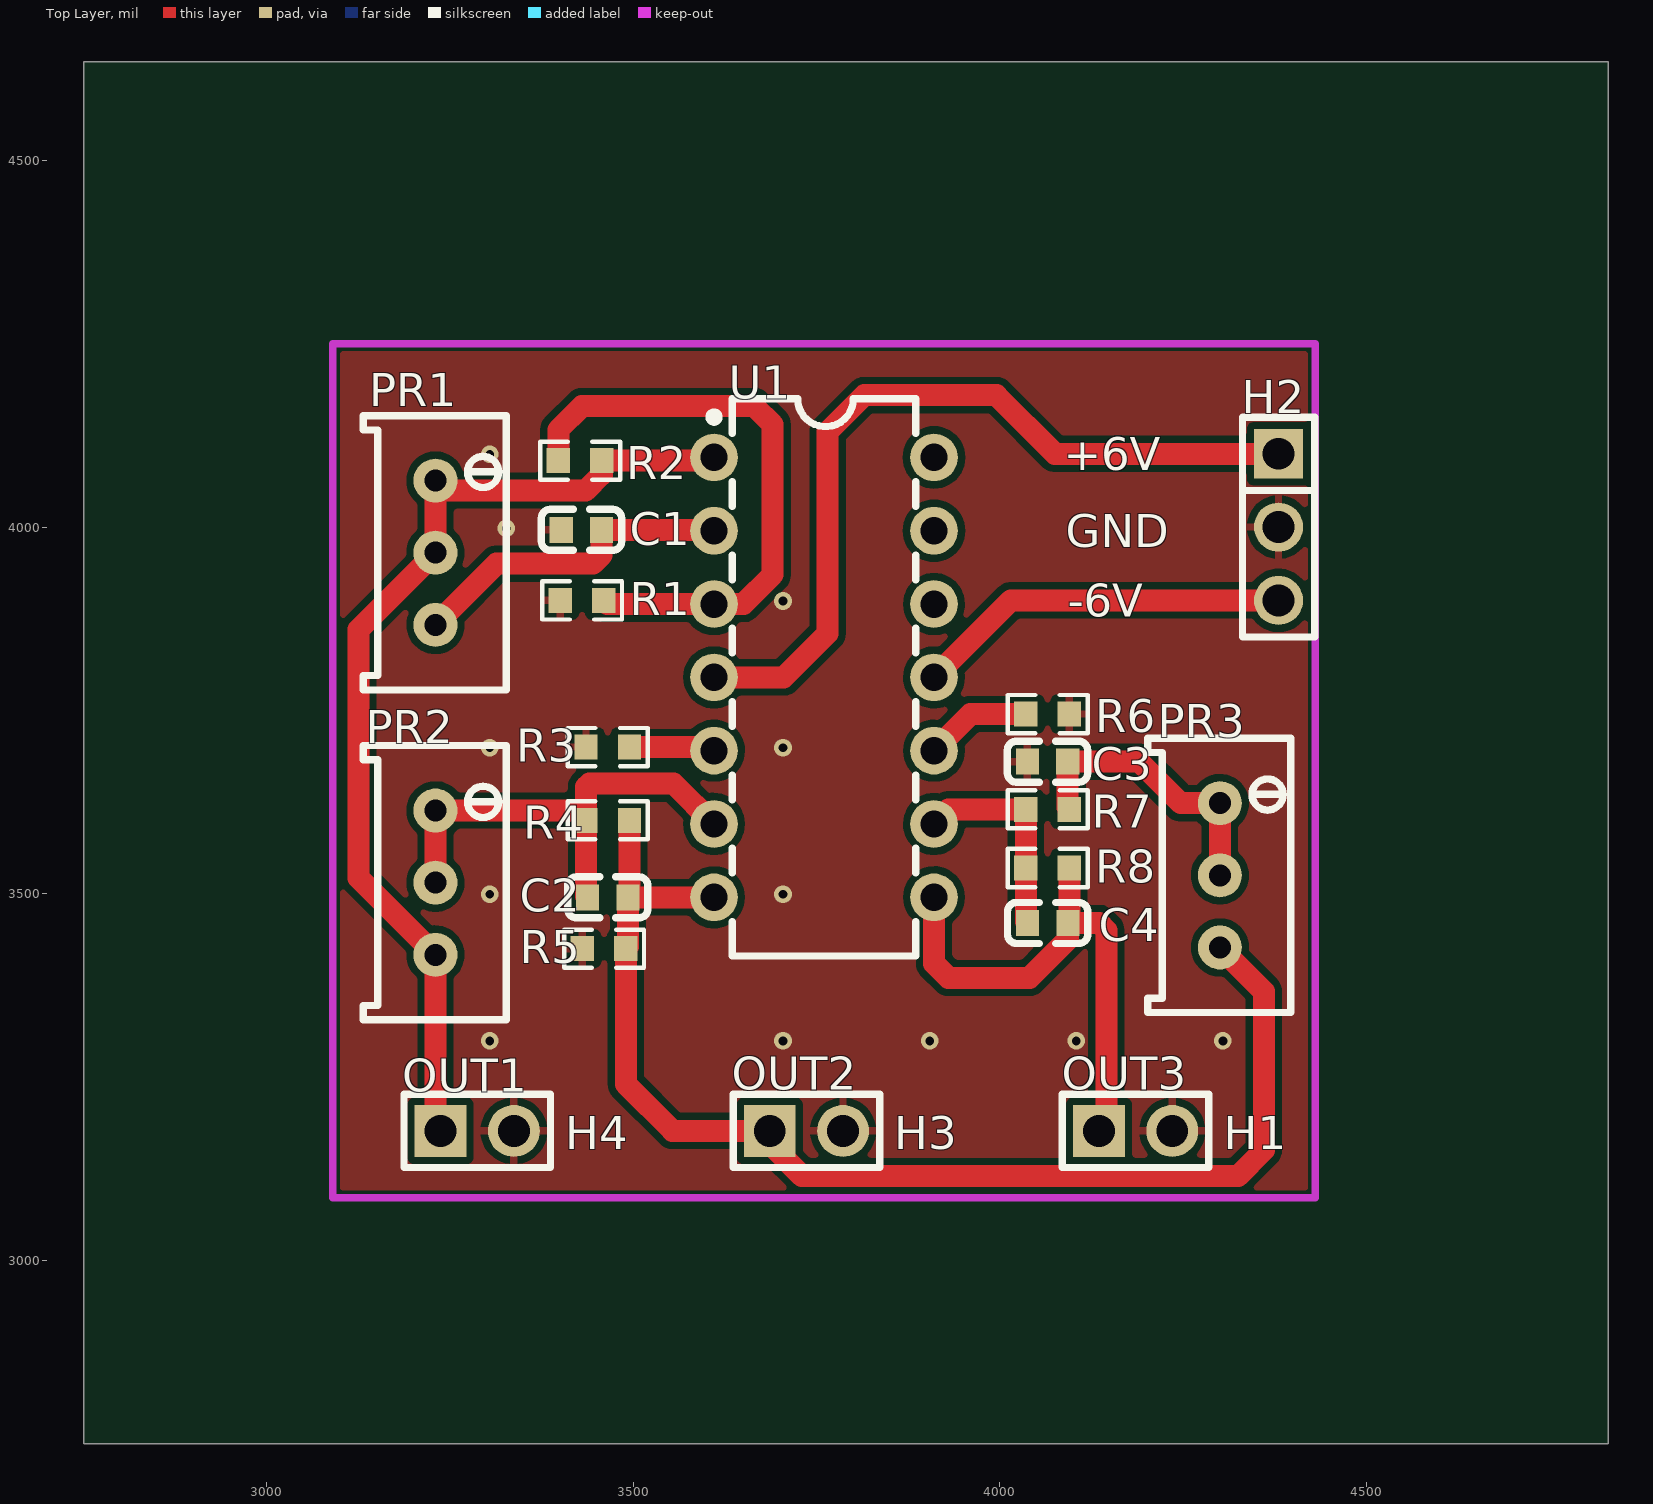
[diagram p0: Top Layer view]
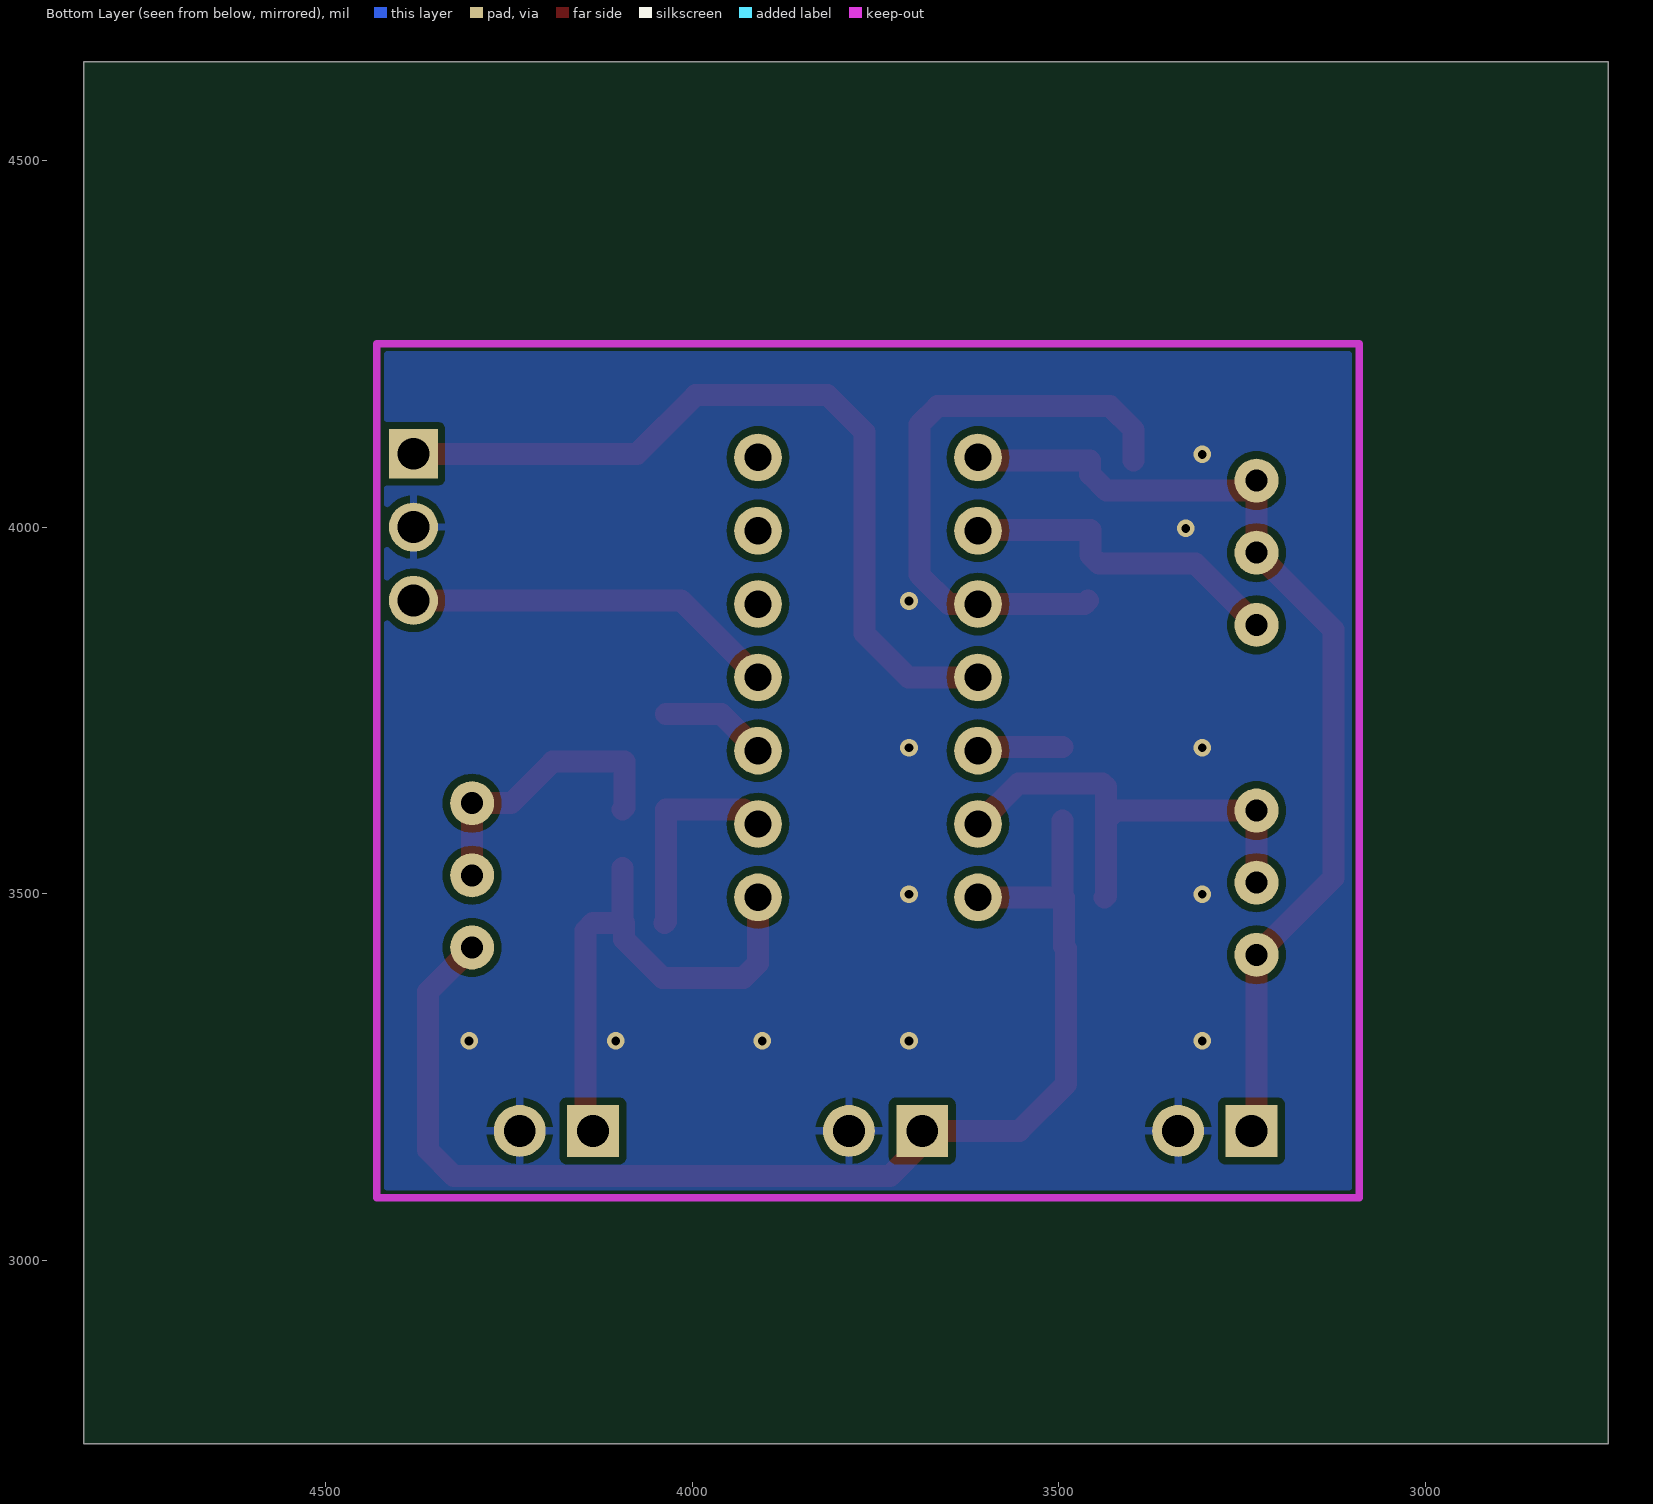
[diagram p1: Bottom Layer view, seen from below]
# Altium PCB MISC51897.pcbdoc
Units mil, origin at the board's own origin, x right, y up, seen from the top; angles counter-clockwise.
Board outline 2080 x 1885 mil, 2 copper layers (Top Layer, Bottom Layer), stack 62.206 mil thick; 20 components, 13 nets, 56 pads, 12 vias.

## Layer stack, top to bottom
Top Solder Mask Layer: solder mask 0.394, Dk 3.3
Top Layer: signal copper 1.379
Dielectric1: surface 59.449, FR4, Dk 4.5
Bottom Layer: signal copper 1.378
Bottom Solder Mask Layer: solder mask 0.394, Dk 3.3

## Board outline
4830,2750 2750,2750 2750,4635 4830,4635

## Design rules (kind name [scope] priority, off if disabled: settings)
BoardOutlineClearance copperThickness2oz_1 [All] p2 off: genericclearance=7.99 ignorepadtopadclearanceinfootprint=FALSE except(0: Arc-SplitContinuation Track-SplitContinuation SMDPad-SplitContinuation THPad-SplitContinuation Via-SplitContinuation Fill-SplitContinuation Region-SplitContinuation Poly-SplitContinuation Text-SplitContinuation Hole-SplitContinuation; 5.98: Arc-CutoutEdge SMDPad-CutoutEdge THPad-CutoutEdge Via-CutoutEdge Fill-CutoutEdge Region-CutoutEdge Text-CutoutEdge; 6.93: Hole-OutlineEdge Hole-CutoutEdge; 10: Poly-OutlineEdge Poly-CutoutEdge; 11.81: Arc-OutlineEdge Track-OutlineEdge SMDPad-OutlineEdge THPad-OutlineEdge Via-OutlineEdge Fill-OutlineEdge Region-OutlineEdge Text-OutlineEdge Track-CutoutEdge)
BoardOutlineClearance copperThickness1oz_1 [All] p4: genericclearance=4.02 ignorepadtopadclearanceinfootprint=FALSE except(0: Arc-SplitContinuation Track-SplitContinuation SMDPad-SplitContinuation THPad-SplitContinuation Via-SplitContinuation Fill-SplitContinuation Region-SplitContinuation Poly-SplitContinuation Text-SplitContinuation Hole-SplitContinuation; 6: SMDPad-CutoutEdge THPad-CutoutEdge Via-CutoutEdge Fill-CutoutEdge Region-CutoutEdge Text-CutoutEdge; 6.93: Hole-OutlineEdge Hole-CutoutEdge; 10: Poly-OutlineEdge Poly-CutoutEdge; 11.8: Arc-OutlineEdge Track-OutlineEdge SMDPad-OutlineEdge THPad-OutlineEdge Via-OutlineEdge Fill-OutlineEdge Region-OutlineEdge Text-OutlineEdge; 11.81: Arc-CutoutEdge Track-CutoutEdge)
Clearance copperThickness2oz [All] p1 off: gap=7.99 ignorepadtopadclearanceinfootprint=FALSE except(5.98: SMDPad-Track SMDPad-SMDPad THPad-Track SMDPad-THPad THPad-THPad Track-Via SMDPad-Via THPad-Via Via-Via Fill-Track Region-Track Fill-SMDPad Region-SMDPad Fill-THPad Region-THPad Fill-Via Region-Via Fill-Fill Fill-Region Region-Region Arc-Track Arc-SMDPad Arc-THPad Arc-Via Fill-Arc Region-Arc Arc-Arc Text-Track SMDPad-Text Text-THPad Text-Via Fill-Text Region-Text Arc-Text Text-Text; 6.93: Hole-Track Hole-SMDPad Hole-THPad Hole-Via Fill-Hole Region-Hole Hole-Arc Hole-Text; 10: Poly-Track Poly-SMDPad Poly-THPad Poly-Via Poly-Fill Poly-Region Poly-Poly Poly-Arc Poly-Text Poly-Hole)
Clearance copperThickness1oz [All] p3: gap=4.02 ignorepadtopadclearanceinfootprint=FALSE except(5.98: SMDPad-Track SMDPad-SMDPad THPad-Track SMDPad-THPad THPad-THPad Track-Via SMDPad-Via THPad-Via Via-Via Fill-Track Region-Track Fill-SMDPad Region-SMDPad Fill-THPad Region-THPad Fill-Via Region-Via Fill-Fill Fill-Region Region-Region; 6: Arc-Track Arc-SMDPad Arc-THPad Arc-Via Fill-Arc Region-Arc Arc-Arc Text-Track SMDPad-Text Text-THPad Text-Via Fill-Text Region-Text Arc-Text Text-Text; 6.93: Hole-Track Hole-SMDPad Hole-THPad Hole-Via Fill-Hole Region-Hole Hole-Arc Hole-Text; 10: Poly-Track Poly-SMDPad Poly-THPad Poly-Via Poly-Fill Poly-Region Poly-Poly Poly-Arc Poly-Text Poly-Hole)
DiffPairsRouting differentialPair [All] p1: maxlimit=6 minlimit=6 mostfreqgap=6 toplayer_minwidth=5 toplayer_prefwidth=10 toplayer_maxwidth=100 toplayer_mingap=6 toplayer_prefgap=6 toplayer_maxgap=6 bottomlayer_minwidth=5 bottomlayer_prefwidth=10 bottomlayer_maxwidth=100 bottomlayer_mingap=6 bottomlayer_prefgap=6 bottomlayer_maxgap=6 maxuncoupledlength=10
HoleToHoleClearance otherClearance [All] p1: gap=11.81 allowstackedmicrovias=TRUE
Length netLength [All] p1: minlimit=0 maxlimit=0
MatchedLengths netLengthTolerance [All] p1: tolerance=1000
PasteMaskExpansion pasteMaskExpansion [All] p1: expansion=0
PlaneConnect innerPlane [All] p1: planeconnectstyle=Relief reliefexpansion=20 reliefentries=4 reliefconductorwidth=10 reliefairgap=10
PolygonConnect copperRegion [(InNet('GND'))] p1: connectstyle=Relief reliefconductorwidth=10 reliefentries=4 polygonreliefangle="90 Angle" airgapwidth=10 via.connectstyle=Relief via.reliefconductorwidth=10 via.reliefentries=4 via.polygonreliefangle="90 Angle" via.airgapwidth=10
RoutingVias viaSize [All] p1: holewidth=12.01 width=24.02 viastyle="Through Hole" minholewidth=11.81 minwidth=19.68 maxholewidth=248.03 maxwidth=393.7
SolderMaskExpansion solderMaskExpansion [IsVia] p1: expansion=-1000 istentingtop=TRUE
SolderMaskExpansion solderMaskExpansion [All] p2: expansion=2 istentingtop=FALSE
Width copperThickness2oz_2 [All] p1 off: maxlimit=100 minlimit=8 preferedwidth=10
Width copperThickness1oz_2 [All] p2: maxlimit=100 minlimit=5 preferedwidth=10

## Components (designator, comment, footprint, x,y, rotation, side; value= is the part's Value field where it differs from the comment)
C1 "30nF" C0603 3429.22,3996.21 r0 top
C2 "100nF" C0603 3465,3495 r0 top
C3 "100nF" C0603 4064.88,3680 r0 top
C4 "100nF" C0603 4065,3460 r0 top
H1 "" HDR-TH_2P-P2.54-V-M-1 4185,3176.4 r0 top
H2 "" HDR-TH_3P-P2.54-V-M 4380,4000 r270 top
H3 "" HDR-TH_2P-P2.54-V-M-1 3736,3176.4 r0 top
H4 "" HDR-TH_2P-P2.54-V-M-1 3287,3176.4 r0 top
PR1 "10kΩ" R_3296 3235,3965 r270 top
PR2 "20kΩ" R_3296 3235,3515 r270 top
PR3 "200kΩ" R_3296 4305,3525 r270 top
R1 "10K" R0603 3430,3900 r0 top
R2 "3.9kΩ" R0603 3427.28,4090.63 r180 top
R3 "100K" R0603 3465,3700 r0 top
R4 "300K" R0603 3465,3600 r0 top
R5 "620" R0603 3460,3425 r0 top
R6 "10K" R0603 4065,3745 r180 top
R7 "20K" R0603 4065,3615 r180 top
R8 "24K" R0603 4065,3535 r0 top
U1 "LM324N/PB" PDIP-14_L19.2-W6.6-P2.54-LS7.6-BL 3760,3795 r270 top

## Footprints (in the part's own frame and the unit in brackets; to place one, negate y for a bottom-side part, rotate by r counter-clockwise, add the part's x,y. Pads: shape width x height; smd on the part's side, far side on the other; paste and mask are expansions set on the pad)
C0603 [mm]
  rect 0.8x0.9 smd: 1(-0.7,0) 2(0.7,0)
  silkscreen extent -1.39,-0.71 1.39,0.71
HDR-TH_2P-P2.54-V-M-1 [mm]
  rect 1.8x1.8 hole 1.1: 1(-1.27,0)
  round 1.8 hole 1.1: 2(1.27,0)
  silkscreen extent -2.54,-1.27 2.54,1.27
HDR-TH_3P-P2.54-V-M [mm]
  rect 1.7x1.7 hole 1.1: 1(-2.54,0)
  round 1.7 hole 1.1: 2(0,0) 3(2.54,0)
  silkscreen extent -3.81,-1.25 3.81,1.25
PDIP-14_L19.2-W6.6-P2.54-LS7.6-BL [mm]
  round 1.65 hole 0.95: 1(-7.62,-3.81) 2(-5.08,-3.81) 3(-2.54,-3.81) 4(0,-3.81) 5(2.54,-3.81) 6(5.08,-3.81) 7(7.62,-3.81) 8(7.62,3.81) 9(5.08,3.81) 10(2.54,3.81) 11(0,3.81) 12(-2.54,3.81) 13(-5.08,3.81) 14(-7.62,3.81)
  silkscreen extent -9.65,-3.96 9.65,3.17
R0603 [mil]
  rect 31.75x34.02 smd paste-3937.01 mask+2: 1(-29.66,0) 2(29.66,0)
  silkscreen extent -55,-26 55,26
R_3296 [mil]
  round 60 hole 30 paste+0 mask+2: 1(-98.4,-5) 2(0,-5) 3(98.4,-5)
  silkscreen extent -187,-103 187,92

## Via types
v1: diameter 24.02, hole 12, Top Layer to Bottom Layer, 12 vias

## Nets (pads, with @x,y where several pads share a name; then routed paths per layer and width w, separated by ;. In a path a pad name is that pad's centre, name@x,y a point inside that pad or via, vN(x,y) a via of type N, cw(c..) or ccw(c..) an arc to the next point about the centre after c; other vN are vias at no path point)
6V: H2.1 U1.4 | length 1123.7
  Top Layer w30: U1.4 3705,3795 3765,3855 3765,4130 3815,4180 3995,4180 4075,4100 H2.1
$1N1: R1.2 R2.2 U1.3 | length 812.1
  Top Layer w30: R2.2 3397.62,4132.62 3430,4165 3665,4165 3690,4140 3690,3935 3650,3895 U1.3 3464.66,3895 R1.2
$1N4: C1.2 PR1.3 U1.2 | length 454.4
  Top Layer w30: PR1.3 3313.4,3950 3445,3950 3456.78,3961.78 C1.2 3608.8,3996.21 U1.2
$1N8: H4.1 PR1.1 PR1.2 PR2.3 R2.1 U1.1 | length 1392
  Top Layer w30: H4.1 3230,3183.4 PR2.3 3125,3521.6 3125,3860 PR1.2 PR1.1 3243.4,4050 3435,4050 3456.94,4071.94 R2.1 3605.63,4090.63 U1.1
$1N9: R3.2 U1.5 | length 117.4
  Top Layer w30: R3.2 3605.01,3700 U1.5
$1N11: C2.2 H3.1 PR3.3 R4.2 R5.2 U1.7 | length 1727.6
  Top Layer w30: R4.2 3494.66,3497.1 C2.2 ; U1.7 C2.2 ; PR3.3 4360,3366.6 4360,3150 4325,3115 3730,3115 3686,3159 H3.1 3553.6,3176.4 3489.66,3240.34 R5.2 3492.56,3427.9 C2.2
$1N12: C2.1 PR2.1 PR2.2 R4.1 U1.6 | length 659.9
  Top Layer w30: PR2.2 PR2.1 3421.94,3613.4 R4.1 ; C2.1 3435.34,3497.1 R4.1 ; U1.6 3555.01,3650 3440,3650 3435.34,3645.34 R4.1
$1N17: R6.2 U1.10 | length 146
  Top Layer w30: U1.10 3960,3745 R6.2
$1N19: C4.1 R7.2 R8.1 U1.9 | length 289.5
  Top Layer w30: U1.9 3930,3615 R7.2 R8.1 4035.34,3462.1 C4.1
$1N20: C3.2 PR3.1 PR3.2 R7.1 | length 395.3
  Top Layer w30: R7.1 4092.44,3617.22 C3.2 4190,3680 4246.6,3623.4 PR3.1 PR3.2
$1N22: C4.2 H1.1 R8.2 U1.8 | length 735.2
  Top Layer w30: U1.8 3910,3405 3930,3385 4040,3385 4092.56,3437.56 C4.2 ; R8.2 4094.66,3462.1 C4.2 ; H1.1 4145,3186.4 4145,3450 4135,3460 C4.2
-6V: H2.3 U1.11 | length 513.5
  Top Layer w30: U1.11 4015,3900 H2.3
GND: C1.1 C3.1 H1.2 H2.2 H3.2 H4.2 R1.1 R3.1 R5.1 R6.1
  other v1: 3304.1,3299.1 3704.1,3299.1 3904.1,3299.1 4104.1,3299.1 4304.1,3299.1 3304.1,3499.1 3704.1,3499.1 3304.1,3699.1 3704.1,3699.1 3704.1,3899.1 3326.5,3998.18 3304.1,4099.1
pads on no net: U1.12 U1.13 U1.14

## Polygon pours and split planes (outlines as drawn)
GND on Top Layer (solid, remove dead copper, pour order 0): 3000,4385 3000,3055 4460,3055 4460,4385
GND on Bottom Layer (solid, remove dead copper, pour order 2): 3010,4370 3010,3000 4580,3000 4580,4370

## Keep-outs
Board Outline Layer:
  lines w10: 3090,3085 3090,4250 4430,4250 4430,3085 3090,3085

## Silkscreen, mask and mechanical layers (free items; w line width, h text height)
Top Silkscreen Layer:
  text "+6V" at 4086.99,4077.5 h45
  text "GND" at 4089.4,3972.5 h45
  text "-6V" at 4092.26,3877.5 h45
  text "OUT2" at 3634.4,3232.5 h45
  text "OUT3" at 4084.4,3232.5 h45
  text "OUT1" at 3185,3230 h45